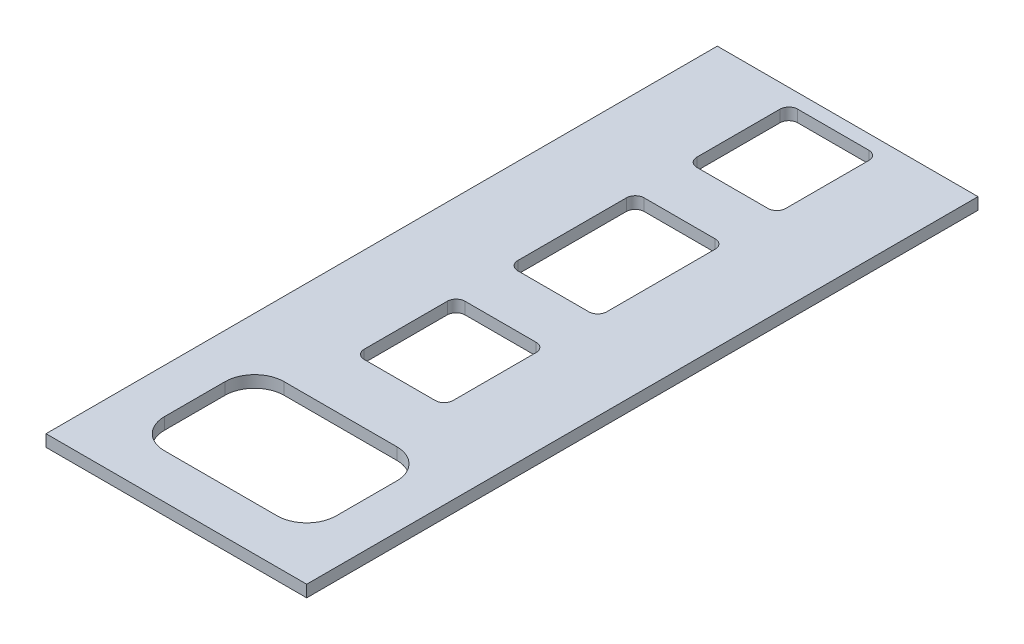
SolidWorks part; units mm, degrees
ref_plane "前视基准面" through (0, 0, 0) normal (0, 0, 1) x (1, 0, 0)
ref_plane "上视基准面" through (0, 0, 0) normal (0, 1, 0) x (1, 0, 0)
ref_plane "右视基准面" through (0, 0, 0) normal (1, 0, 0) x (0, 0, -1)
sketch "草图1" plane through (0, 0, 0) normal (0, 1, 0) x (1, 0, 0)
  line L1 (-440, -1133) -> (440, -1133)
  line L2 (-440, -1133) -> (-440, 1133)
  line L3 (-440, 1133) -> (440, 1133)
  line L4 (440, -1133) -> (440, 1133)
  line L5 (-440, -1133) -> (440, 1133) construction
  line L6 (-440, 1133) -> (440, -1133) construction
  point P0 (0, 0)
  dimension "D1" = 880
  dimension "D2" = 2266
extrude "凸台-拉伸1" add sketch "草图1" along normal blind 40
sketch "草图2" plane through (0, 0, 0) normal (0, -1, 0) x (1, 0, 0)
  line L0 (440, 1133) -> (440, -1133) construction
  line L1 (-150, 378.9847) -> (150, 378.9847)
  line L2 (-150, 378.9847) -> (-150, 38.5153)
  line L3 (-150, 38.5153) -> (150, 38.5153)
  line L4 (150, 378.9847) -> (150, 38.5153)
  dimension "D1" = 290
  dimension "D2" = 590
  dimension "D3" = 1171.5153
  dimension "D4" = 1511.9847
extrude "切除-拉伸1" cut sketch "草图2" against normal through all
sketch "草图3" plane through (0, 0, 0) normal (0, -1, 0) x (1, 0, 0)
  line L0 (150, 38.5153) -> (150, 378.9847) construction
  line L1 (-150, -566.0153) -> (150, -566.0153)
  line L2 (-150, -566.0153) -> (-150, -139.4847)
  line L3 (-150, -139.4847) -> (150, -139.4847)
  line L4 (150, -566.0153) -> (150, -139.4847)
  point P4 (-150, -109.4847)
  point P5 (150, -566.0153)
  point P8 (-150, -139.4847)
  dimension "D1" = 300
  dimension "D2" = 178
  dimension "D3" = 604.5306
extrude "切除-拉伸2" cut sketch "草图3" against normal through all
sketch "草图4" plane through (0, 0, 0) normal (0, -1, 0) x (-1, 0, 0)
  line L0 (-150, 566.0153) -> (-150, 139.4847) construction
  line L1 (150, 744.0153) -> (-150, 744.0153)
  line L2 (150, 744.0153) -> (150, 1084.4847)
  line L3 (150, 1084.4847) -> (-150, 1084.4847)
  line L4 (-150, 744.0153) -> (-150, 1084.4847)
  line L6 (-150, 139.4847) -> (150, 139.4847) construction
  point P4 (150, 744.0153)
  point P5 (150, 1084.4847)
  dimension "D1" = 300
  dimension "D2" = 604.5306
  dimension "D3" = 945
extrude "切除-拉伸3" cut sketch "草图4" against normal through all
sketch "草图5" plane through (0, 0, 0) normal (0, -1, 0) x (1, 0, 0)
  line L0 (-440, 1133) -> (440, 1133) construction
  line L1 (-290, 983) -> (290, 983)
  line L2 (-290, 983) -> (-290, 578.9847)
  line L3 (-290, 578.9847) -> (290, 578.9847)
  line L4 (290, 983) -> (290, 578.9847)
  line L5 (440, 1133) -> (440, -1133) construction
  line L6 (-440, -1133) -> (-440, 1133) construction
  line L7 (150, 378.9847) -> (-150, 378.9847) construction
  dimension "D1" = 150
  dimension "D2" = 150
  dimension "D3" = 150
  dimension "D4" = 200
extrude "切除-拉伸4" cut sketch "草图5" against normal through all
fillet "圆角2" radius 100 4 edges at (290, 20, 983) (290, 20, 578.9847) (-290, 20, 578.9847) (-290, 20, 983)
fillet "圆角3" radius 30 12 edges at (150, 20, 378.9847) (150, 20, 38.5153) (-150, 20, 38.5153) (150, 20, -139.4847) (150, 20, -566.0153) (-150, 20, -566.0153) (-150, 20, -139.4847) (150, 20, -744.0153) (150, 20, -1084.4847) (-150, 20, -1084.4847) (-150, 20, -744.0153) (-150, 20, 378.9847)
